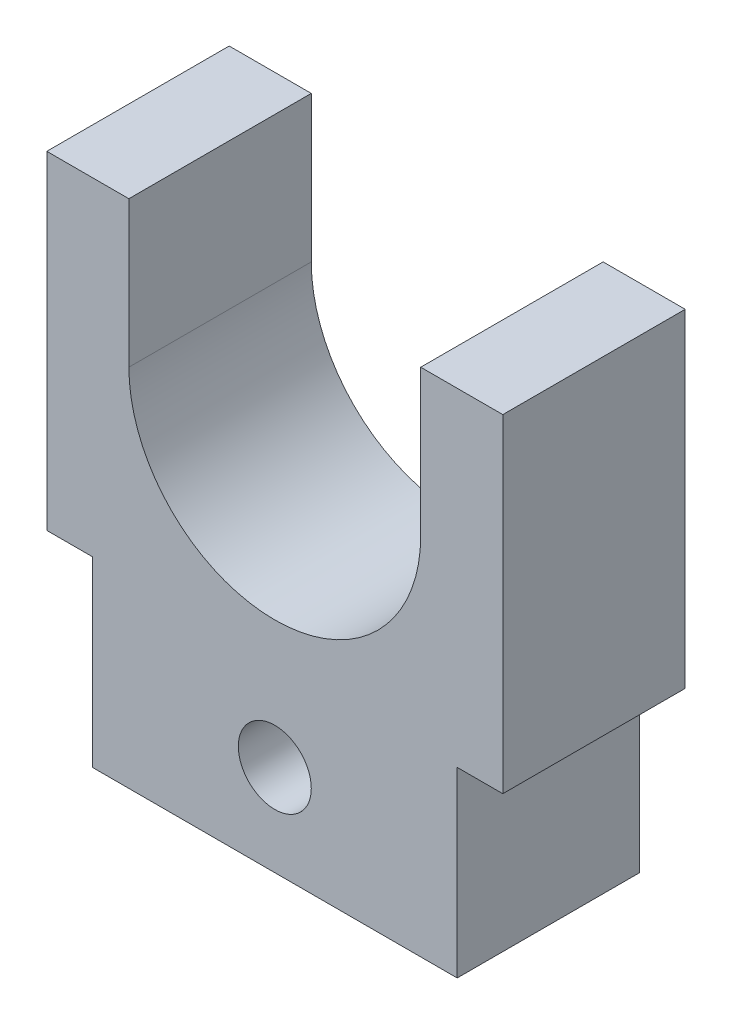
SolidWorks part; units mm, degrees
ref_plane "前视基准面" through (0, 0, 0) normal (0, 0, 1) x (1, 0, 0)
ref_plane "上视基准面" through (0, 0, 0) normal (0, 1, 0) x (1, 0, 0)
ref_plane "右视基准面" through (0, 0, 0) normal (1, 0, 0) x (0, 0, -1)
sketch "草图1" plane through (0, 0, 0) normal (0, 0, 1) x (1, 0, 0)
  line L0 (0, 10) -> (-2.5, 10)
  line L1 (0, 0) -> (20, 0)
  line L2 (0, 0) -> (0, 10)
  line L3 (18, 20) -> (18, 28)
  line L4 (20, 0) -> (20, 10)
  line L5 (-2.5, 10) -> (-2.5, 27.1421)
  line L7 (20, 10) -> (22.5, 10)
  line L8 (22.5, 10) -> (22.5, 28)
  line L9 (18, 28) -> (22.5, 28)
  line L10 (2, 20) -> (2, 28)
  line L11 (2, 28) -> (-2.5, 28)
  line L12 (-2.5, 28) -> (-2.5, 27.1421)
  circle A0 centre (10, 5) radius 2
  arc A1 (2, 20) -> (18, 20) centre (10, 20) ccw
  dimension "D1" = 5
  dimension "D2" = 15
  dimension "D3" = 10
  dimension "D4" = 10
extrude "凸台-拉伸1" add sketch "草图1" along normal blind 10
